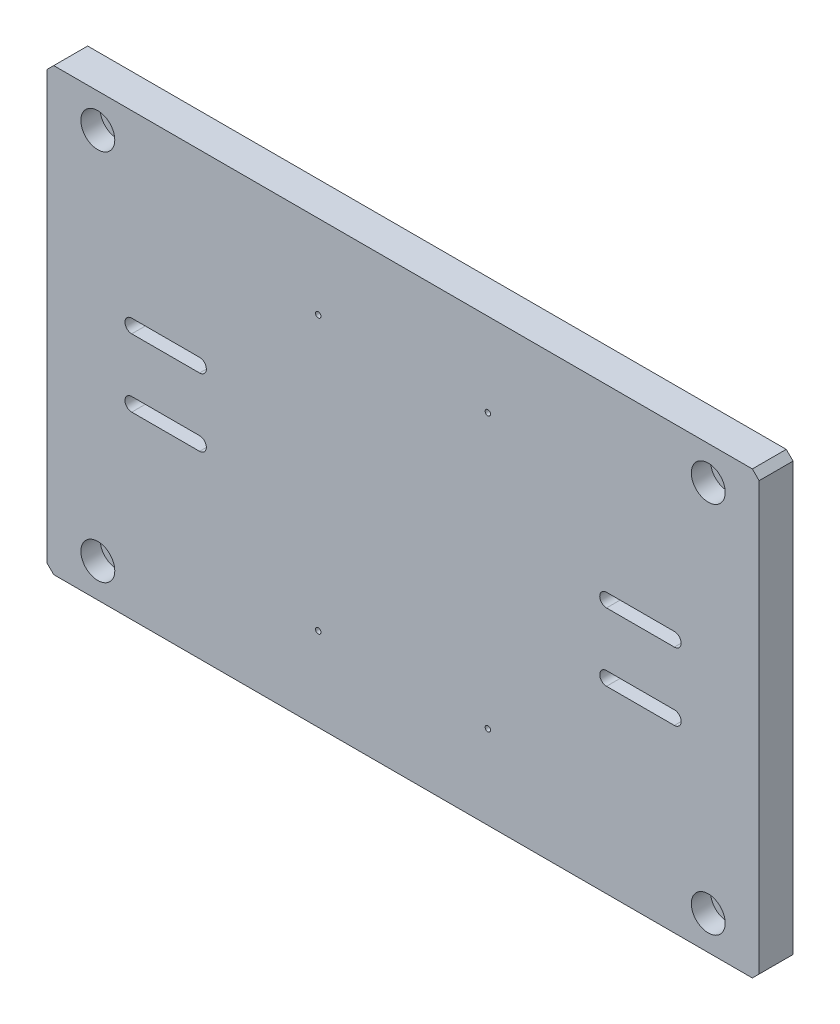
from build123d import *

# Parameters (mm, degrees)
SKETCH1_W                                           = 210
SKETCH1_H                                           = 130
BOSS_EXTRUDE1_DEPTH                                 = 10
CUT_EXTRUDE1_DEPTH                                  = 124.895116934
CUT_EXTRUDE1_DEPTH_BACK                             = 124.895116934
HOLE_SIZE_PER_SOCKET_HEAD_CAP_SCREW_TYP_D           = 5.5
HOLE_SIZE_PER_SOCKET_HEAD_CAP_SCREW_TYP_CBORE_D     = 10
HOLE_SIZE_PER_SOCKET_HEAD_CAP_SCREW_TYP_CBORE_DEPTH = 5.7
M2_TAPPED_HOLE1_D                                   = 1.6
CHAMFER1_SIZE                                       = 2


with BuildPart() as part:
    # Sketch1 → Boss-Extrude1 (new body)
    with BuildSketch(Plane.XY):
        Rectangle(SKETCH1_W, SKETCH1_H)
    extrude(amount=BOSS_EXTRUDE1_DEPTH)

    # Sketch2 → Cut-Extrude1 (cut, two sides: drawn at the far end of the back side and taken through both)
    with BuildSketch(Plane.XY.offset(10).offset(-CUT_EXTRUDE1_DEPTH_BACK)):
        with BuildLine():
            Line((-80, 8), (-60, 8))
            ThreePointArc((-60, 8), (-58, 10), (-60, 12))
            Line((-60, 12), (-80, 12))
            ThreePointArc((-80, 12), (-82, 10), (-80, 8))
        make_face()
        with BuildLine():
            ThreePointArc((-60, -8), (-58, -10), (-60, -12))
            Line((-60, -12), (-80, -12))
            ThreePointArc((-80, -12), (-82, -10), (-80, -8))
            Line((-80, -8), (-60, -8))
        make_face()
        with BuildLine():
            Line((80, -8), (60, -8))
            ThreePointArc((60, -8), (58, -10), (60, -12))
            Line((60, -12), (80, -12))
            ThreePointArc((80, -12), (82, -10), (80, -8))
        make_face()
        with BuildLine():
            Line((80, 12), (60, 12))
            ThreePointArc((60, 12), (58, 10), (60, 8))
            Line((60, 8), (80, 8))
            ThreePointArc((80, 8), (82, 10), (80, 12))
        make_face()
    extrude(amount=CUT_EXTRUDE1_DEPTH + CUT_EXTRUDE1_DEPTH_BACK, mode=Mode.SUBTRACT)

    # Hole size (per socket head cap screw type)1 (through all)
    with Locations(Plane(origin=(-90, 55, 10), x_dir=(1, 0, 0), z_dir=(0, 0, 1))):
        with Locations((0, 0), (0, -110), (180, -110), (180, 0)):
            CounterBoreHole(HOLE_SIZE_PER_SOCKET_HEAD_CAP_SCREW_TYP_D / 2, HOLE_SIZE_PER_SOCKET_HEAD_CAP_SCREW_TYP_CBORE_D / 2, HOLE_SIZE_PER_SOCKET_HEAD_CAP_SCREW_TYP_CBORE_DEPTH)

    # M2 Tapped Hole1 (through all)
    with Locations(Plane(origin=(-25, 40.35, 10), x_dir=(1, 0, 0), z_dir=(0, 0, 1))):
        with Locations((0, 0), (50, 0), (50, -80.7), (0, -80.7)):
            Hole(M2_TAPPED_HOLE1_D / 2)

    # Chamfer1
    chamfer1_edges = [part.edges().sort_by_distance(p)[0] for p in [
        (105, -65, 5),
        (-105, -65, 5),
        (-105, 65, 5),
        (105, 65, 5),
    ]]
    chamfer(chamfer1_edges, length=CHAMFER1_SIZE)


solid = part.part
